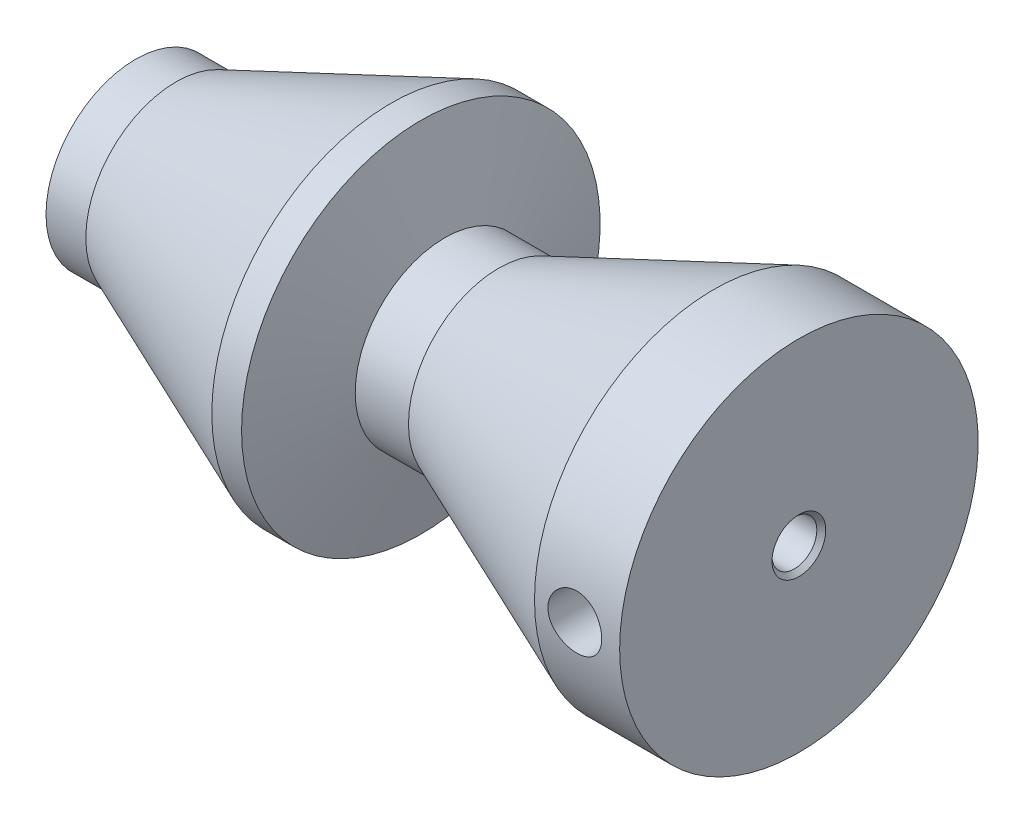
from build123d import *

# Parameters (mm, degrees)
HOLE_WIZARD_M6_1_D        = 5
HOLE_WIZARD_M6_1_DEPTH    = 17
HOLE_WIZARD_M6_1_TIP      = 1.502151548
CHAMFER_1_SIZE            = 0.5
HOLE_WIZARD_6_0_6_1_D     = 6
HOLE_WIZARD_6_0_6_1_DEPTH = 10
HOLE_WIZARD_6_0_6_1_TIP   = 1.802581857


with BuildPart() as part:
    # 草图1 → 旋转1 (revolve)
    with BuildSketch(Plane.XY, mode=Mode.PRIVATE) as revolve_1_sk:
        Polygon((4.5, 10), (0, 10), (0, 0), (74, 0), (74, 20), (64.5, 20), (40.5, 10.058874503), (40.5, 10), (34.5, 10), (31.820508076, 20), (28.5, 20), (4.5, 10.058874503), align=None)
    revolve(revolve_1_sk.sketch.rotate(Axis((0, 0, 0), (1, 0, 0)), 90), axis=Axis((0, 0, 0), (1, 0, 0)))

    # M6 螺纹孔1
    with Locations(Plane(origin=(74, 0, 0), x_dir=(0, 0, -1), z_dir=(1, 0, 0))):
        with Locations((0, 0)):
            Hole(HOLE_WIZARD_M6_1_D / 2, depth=HOLE_WIZARD_M6_1_DEPTH)
            with Locations((0, 0, -(HOLE_WIZARD_M6_1_DEPTH + HOLE_WIZARD_M6_1_TIP / 2))):  # 118° drill point
                Cone(0, HOLE_WIZARD_M6_1_D / 2, HOLE_WIZARD_M6_1_TIP, mode=Mode.SUBTRACT)

    # 倒角1
    chamfer_1_edges = [part.edges().sort_by_distance(p)[0] for p in [
        (74, 0, -2.5),
    ]]
    chamfer(chamfer_1_edges, length=CHAMFER_1_SIZE)

    # Ø6.0 (6) 直径孔1
    with Locations(Plane(origin=(69, 0, 20), x_dir=(1, 0, 0), z_dir=(0, 0, 1))):
        with Locations((0, 0)):
            Hole(HOLE_WIZARD_6_0_6_1_D / 2, depth=HOLE_WIZARD_6_0_6_1_DEPTH)
            with Locations((0, 0, -(HOLE_WIZARD_6_0_6_1_DEPTH + HOLE_WIZARD_6_0_6_1_TIP / 2))):  # 118° drill point
                Cone(0, HOLE_WIZARD_6_0_6_1_D / 2, HOLE_WIZARD_6_0_6_1_TIP, mode=Mode.SUBTRACT)


solid = part.part
